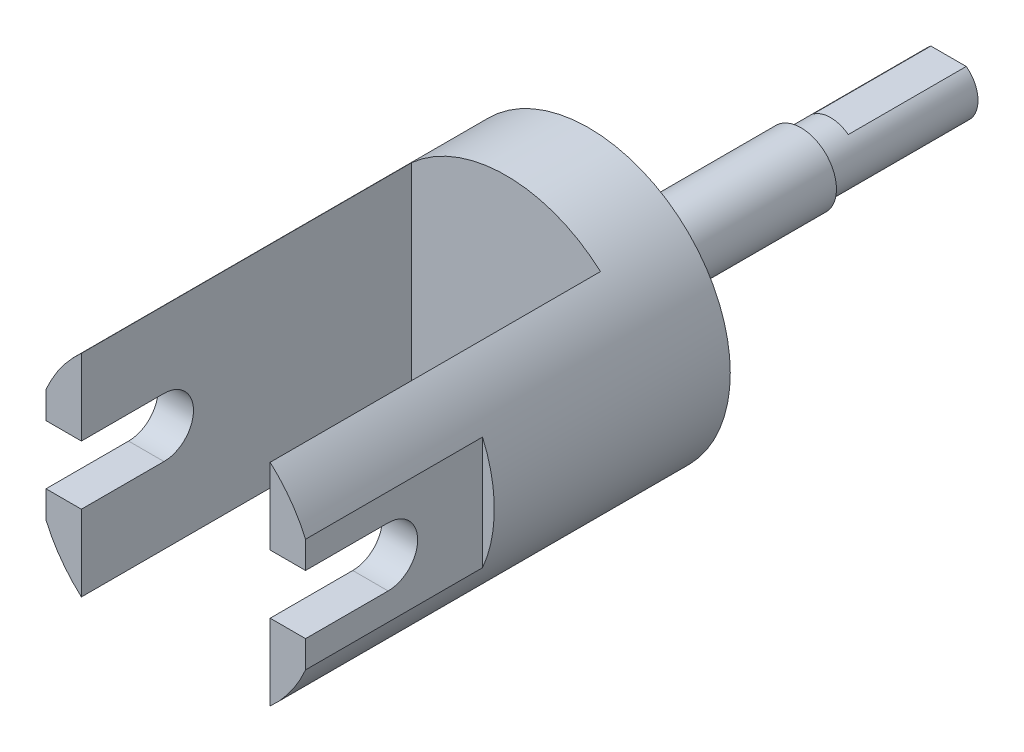
from build123d import *

# Parameters (mm, degrees)
SKETCH1_R           = 12
BOSS_EXTRUDE1_DEPTH = 35
SKETCH2_R           = 3.5
BOSS_EXTRUDE2_DEPTH = 5
SKETCH3_W           = 16
SKETCH3_H           = 25
CUT_EXTRUDE1_DEPTH  = 28
CUT_EXTRUDE2_DEPTH  = 15
CUT_EXTRUDE3_START  = -15
CUT_EXTRUDE3_DEPTH  = 15
SKETCH6_R           = 3
BOSS_EXTRUDE3_DEPTH = 13
SKETCH7_R           = 2.5
BOSS_EXTRUDE4_DEPTH = 12.5
SKETCH8_W           = 9.031547502
SKETCH8_H           = 2.523978301
CUT_EXTRUDE4_DEPTH  = 10


with BuildPart() as part:
    # Sketch1 → Boss-Extrude1 (new body)
    with BuildSketch(Plane.XY):
        Circle(SKETCH1_R)
    extrude(amount=BOSS_EXTRUDE1_DEPTH)

    # Sketch2 → Boss-Extrude2 (add)
    with BuildSketch(Plane(origin=(0, 0, 0), x_dir=(-1, 0, 0), z_dir=(0, 0, -1))):
        Circle(SKETCH2_R)
    extrude(amount=BOSS_EXTRUDE2_DEPTH)

    # Sketch3 → Cut-Extrude1 (cut)
    with BuildSketch(Plane.XY.offset(35)):
        Rectangle(SKETCH3_W, SKETCH3_H)
    extrude(amount=-CUT_EXTRUDE1_DEPTH, mode=Mode.SUBTRACT)

    # Sketch4 → Cut-Extrude2 (cut, symmetric)
    with BuildSketch(Plane(origin=(0, 0, 0), x_dir=(0, 0, -1), z_dir=(1, 0, 0))):
        with BuildLine():
            Line((-28, -2.5), (-35, -2.5))
            Line((-35, -2.5), (-35, 2.5))
            Line((-35, 2.5), (-28, 2.5))
            ThreePointArc((-28, 2.5), (-25.5, 0), (-28, -2.5))
        make_face()
    extrude(amount=CUT_EXTRUDE2_DEPTH, both=True, mode=Mode.SUBTRACT)

    # Sketch5 → Cut-Extrude3 (cut)
    with BuildSketch(Plane.XY.offset(35).offset(CUT_EXTRUDE3_START)):
        with BuildLine():
            Line((11, -4.795831523), (11, 4.795831523))
            ThreePointArc((11, 4.795831523), (12, 0), (11, -4.795831523))
        make_face()
        with BuildLine():
            Line((-11, -4.795831523), (-11, 4.795831523))
            ThreePointArc((-11, 4.795831523), (-12, 0), (-11, -4.795831523))
        make_face()
    extrude(amount=CUT_EXTRUDE3_DEPTH, mode=Mode.SUBTRACT)

    # Sketch6 → Boss-Extrude3 (add)
    with BuildSketch(Plane(origin=(0, 0, -5), x_dir=(-1, 0, 0), z_dir=(0, 0, -1))):
        with Locations(Location((0, 0, 0), (0, 0, 180))):
            Circle(SKETCH6_R)
    extrude(amount=BOSS_EXTRUDE3_DEPTH)

    # Sketch7 → Boss-Extrude4 (add)
    with BuildSketch(Plane(origin=(0, 0, -18), x_dir=(-1, 0, 0), z_dir=(0, 0, -1))):
        Circle(SKETCH7_R)
    extrude(amount=BOSS_EXTRUDE4_DEPTH)

    # Sketch8 → Cut-Extrude4 (cut)
    with BuildSketch(Plane(origin=(0, 0, -30.5), x_dir=(-1, 0, 0), z_dir=(0, 0, -1))):
        with Locations((0, 3.261989151)):
            Rectangle(SKETCH8_W, SKETCH8_H)
    extrude(amount=-CUT_EXTRUDE4_DEPTH, mode=Mode.SUBTRACT)


solid = part.part
